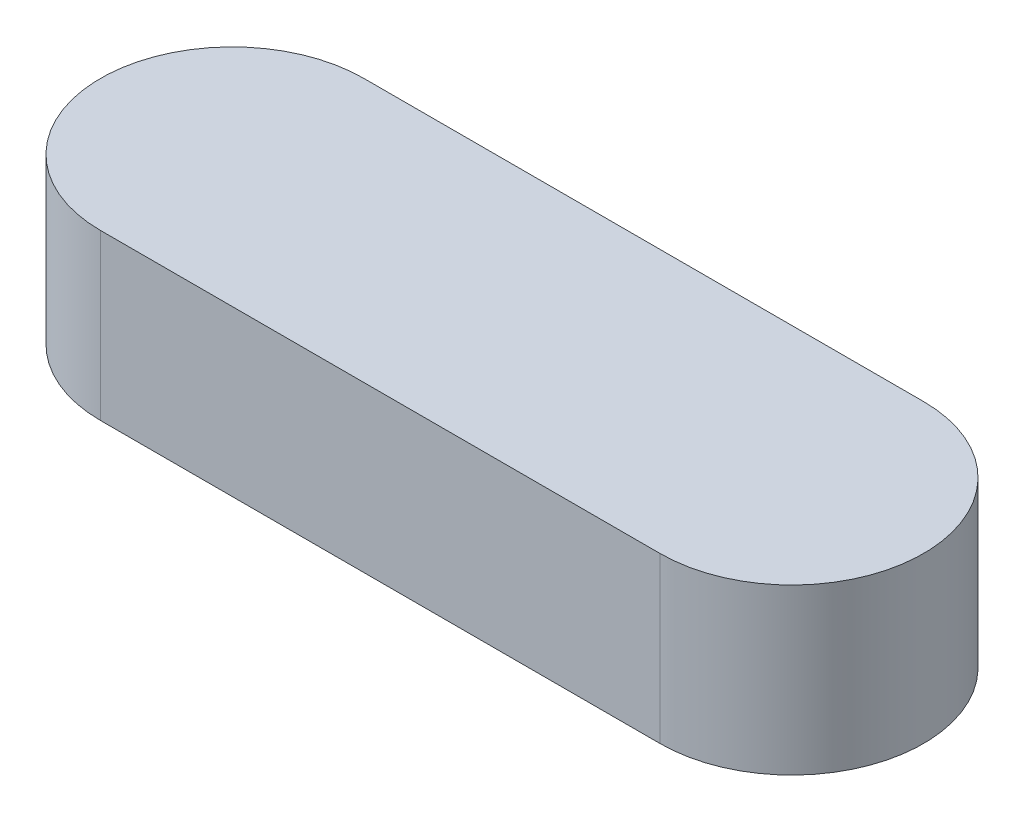
from build123d import *

# Parameters (mm, degrees)
BOSS_EXTRUDE1_DEPTH = 10


with BuildPart() as part:
    # Sketch1 → Boss-Extrude1 (new body)
    with BuildSketch(Plane(origin=(0, 0, 0), x_dir=(1, 0, 0), z_dir=(0, 1, 0))):
        with BuildLine():
            Line((0, 8), (34, 8))
            ThreePointArc((34, 8), (42, 0), (34, -8))
            Line((34, -8), (0, -8))
            ThreePointArc((0, -8), (-8, 0), (0, 8))
        make_face()
    extrude(amount=BOSS_EXTRUDE1_DEPTH)


solid = part.part
